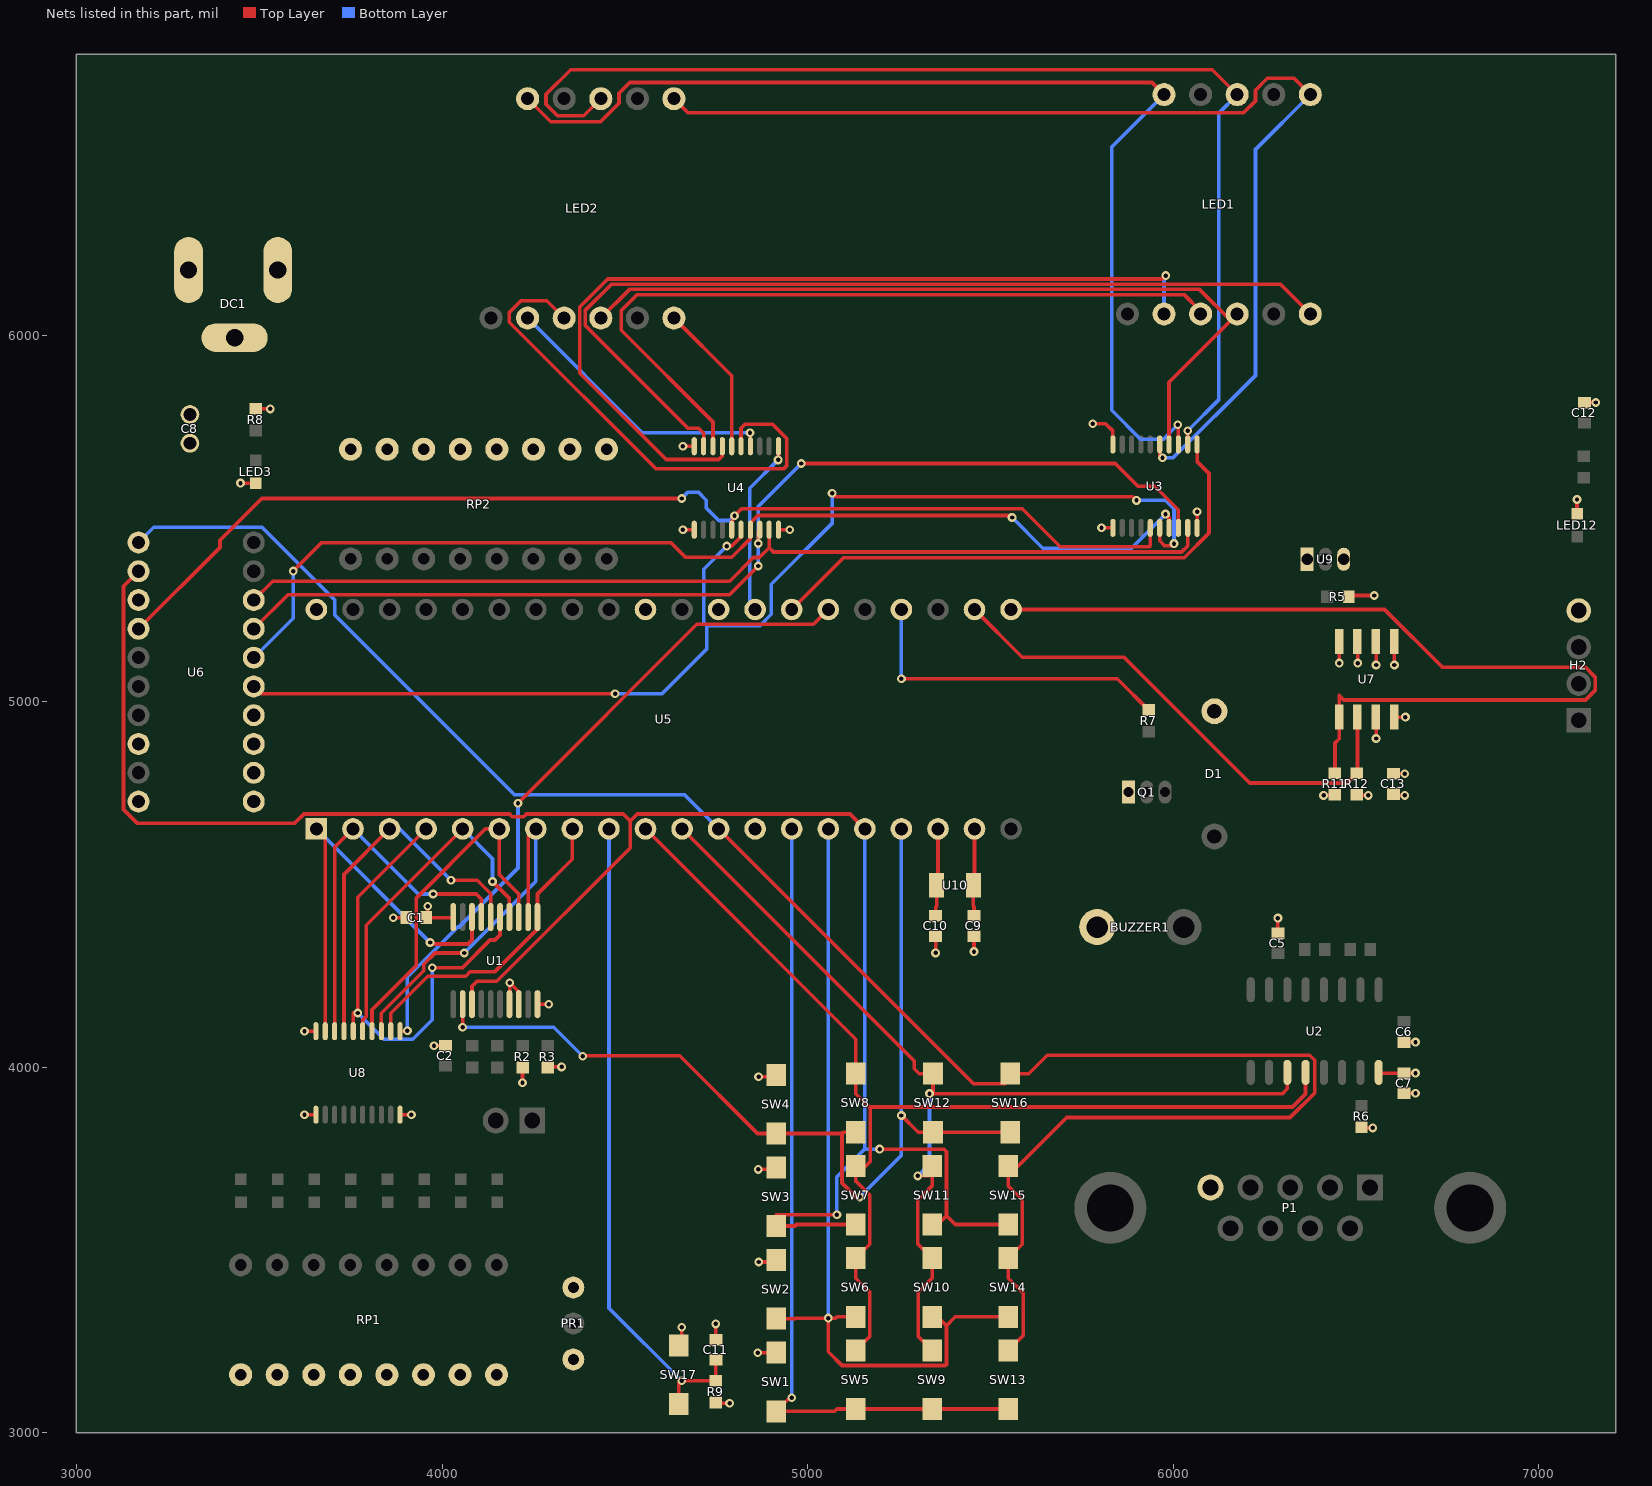
[diagram p0: the nets of this part, all layers, seen from the top]
# Altium PCB MISC49866.pcbdoc (part 2 of 2)
Units mil, origin at the board's own origin, x right, y up, seen from the top; angles counter-clockwise.
Board outline 4210 x 3770 mil, 4 copper layers (Top Layer, Inner1, Inner2, Bottom Layer), stack 62.447 mil thick; 74 components, 100 nets, 357 pads, 104 vias.

## Via types
v1: diameter 24.02, hole 12, Top Layer to Bottom Layer, 104 vias

## Nets (pads, with @x,y where several pads share a name; then routed paths per layer and width w, separated by ;. In a path a pad name is that pad's centre, name@x,y a point inside that pad or via, vN(x,y) a via of type N, cw(c..) or ccw(c..) an arc to the next point about the centre after c; other vN are vias at no path point) (continued)
D3: U3.5 U4.5 U6.4 | length 3125.9
  Top Layer w10: U6.4@3170.04,5198.78 3392.72,5421.46 3392.72,5440.84 3507.3,5555.42 v1(4655.68,5555.42) ; U4.5@4792.36,5470 4792.36,5493.47 4800.03,5501.14 v1(4800.03,5507.98) 4819.15,5527.1 5587.1,5527.1 5691.01,5423.19 5934.85,5423.19 5937.36,5425.7 U3.5@5937.36,5475
  Bottom Layer w10: v1(4655.68,5555.42) 4673.06,5572.8 4700.92,5572.8 4723.08,5550.64 4723.08,5529.42 4757.24,5495.26 4787.31,5495.26 v1(4800.03,5507.98)
D4: U3.6 U4.6 U6.16 | length 3399
  Top Layer w10: U6.16@3485,5041.3 3505.22,5021.08 v1(4473.36,5021.08) ; v1(4779.08,5425.08) 4792.6,5425.08 4817.95,5450.43 U4.6@4817.95,5470 ; v1(5066.96,5569.86) 5076.38,5560.44 5889.43,5560.44 v1(5899.63,5550.16) ; U3.6@5962.95,5475 5962.95,5439.47 5976.72,5425.7 5995.88,5425.7 v1(6002.2,5432.02)
  Bottom Layer w10: v1(4473.36,5021.08) 4601.64,5021.08 4724.33,5143.77 4724.33,5207.49 ; v1(4779.08,5425.08) 4715.87,5361.87 4715.87,5215.95 4724.33,5207.49 ; v1(5066.96,5569.86) 5066.96,5486.96 4900.83,5320.83 4900.83,5238.43 4869.89,5207.49 4724.33,5207.49 ; v1(5899.63,5550.16) 5978.97,5550.16 6002.2,5526.93 v1(6002.2,5432.02)
D5: U3.7 U4.7 U6.15 | length 2905.5
  Top Layer w10: v1(3592.89,5356.8) 3669.98,5433.89 4626.85,5433.89 4665.79,5394.95 4792.72,5394.95 4843.54,5445.77 U4.7@4843.54,5470 4843.54,5488.99 4863.49,5508.94 5553.83,5508.94 v1(5559.36,5503.41) ; v1(5979.04,5512.54) 5988.54,5503.04 U3.7@5988.54,5475
  Bottom Layer w10: U6.15@3485,5120.04 3592.89,5227.93 v1(3592.89,5356.8) ; v1(5559.36,5503.41) 5643.51,5419.26 5885.76,5419.26 v1(5979.04,5512.54)
D6: U3.8 U4.8 U6.14 | length 2953.3
  Top Layer w10: U6.14@3485,5198.78 3578.59,5292.37 4786.35,5292.37 v1(4864.8,5370.82) ; v1(4864.8,5432.12) 4864.8,5465.67 U4.8@4869.13,5470 ; v1(4982.54,5651.13) 5841.27,5651.13 5903.59,5588.81 5949.61,5588.81 6014.13,5524.3 U3.8@6014.13,5475
  Bottom Layer w10: v1(4864.8,5370.82) v1(4864.8,5432.12) 4864.8,5533.4 v1(4982.54,5651.13)
D7: U3.9 U4.9 U6.13 | length 2724.5
  Top Layer w10: U6.13@3485,5277.52 3536.73,5329.25 4786.89,5329.25 4851.62,5393.98 4868,5393.98 4894.72,5420.7 ; U4.9@4894.72,5470 4894.72,5420.7 ; U3.9@6039.72,5475 6039.72,5425.7 6022.88,5408.86 4906.56,5408.86 4894.72,5420.7
DB1: U1.18 U5.1 U8.19 | length 1186.6
  Top Layer w10: U5.1@3656.56,4651.69 3680.59,4627.66 U8.19@3680.59,4098.35 ; v1(3967.37,4340.88) 3971.44,4336.81 4071.19,4336.81 4082.03,4347.65 U1.18@4082.03,4410.54
  Bottom Layer w10: U5.1@3656.56,4651.69 v1(3967.37,4340.88)
DB2: U1.17 U5.2 U8.18 | length 1053.9
  Top Layer w10: U8.18@3706.18,4098.35 3706.18,4601.31 U5.2@3756.56,4651.69 ; v1(3975.6,4473.42) 4093.85,4473.42 4107.62,4459.65 U1.17@4107.62,4410.54
  Bottom Layer w10: U5.2@3756.56,4651.69 3934.83,4473.42 v1(3975.6,4473.42)
DB3: U1.16 U5.3 U8.17 | length 1019.1
  Top Layer w10: U8.17@3731.77,4098.35 3731.77,4526.9 U5.3@3856.56,4651.69 ; v1(4024.51,4511.2) 4096.54,4511.2 4133.21,4474.53 U1.16@4133.21,4410.54
  Bottom Layer w10: U5.3@3856.56,4651.69 3884.02,4651.69 v1(4024.51,4511.2)
DB4: U1.15 U5.4 U8.16 | length 1312.6
  Top Layer w10: U8.16@3757.36,4098.35 3757.36,4147.65 3757.73,4148.02 v1(3769.45,4148.02) 3769.45,4464.58 U5.4@3956.56,4651.69 ; v1(3973.41,4272.07) 4056.01,4272.07 4131.59,4347.65 4145.04,4347.65 4158.81,4361.42 U1.15@4158.8,4410.54
  Bottom Layer w10: v1(3769.45,4148.02) 3841.23,4076.24 3920.25,4076.24 3973.41,4129.4 v1(3973.41,4272.07)
DB5: U1.14 U5.5 U8.15 | length 960.8
  Top Layer w10: U8.15@3782.95,4098.35 3782.95,4128.76 3792.61,4138.42 3792.61,4387.74 U5.5@4056.56,4651.69 ; v1(4138.1,4507.63) 4184.4,4461.34 U1.14@4184.39,4410.54
  Bottom Layer w10: U5.5@4056.56,4651.69 4138.1,4570.15 v1(4138.1,4507.63)
DB6: U1.13 U5.6 U8.14 | length 982.8
  Top Layer w10: U8.14@3808.54,4098.35 3808.54,4157.09 3929.94,4278.49 3929.94,4462.63 4119,4651.69 U5.6@4156.56,4651.69 4156.56,4526.85 4209.98,4473.42 U1.13@4209.98,4410.54
DB7: U1.12 U5.7 U8.13 | length 1025
  Top Layer w10: U8.13@3834.13,4098.35 3834.13,4147.65 3950.25,4263.77 3950.25,4281.66 3980.86,4312.27 v1(4060.88,4312.27) ; U1.12@4235.57,4410.54 4235.57,4630.71 U5.7@4256.56,4651.69
  Bottom Layer w10: v1(4060.88,4312.27) 4256.55,4507.95 U5.7@4256.56,4651.69
DB8: U1.11 U5.8 U8.12 | length 859.5
  Top Layer w10: U8.12@3859.72,4098.35 3859.72,4147.65 3960.98,4248.91 4064.81,4248.91 4077.24,4261.34 4144.77,4261.34 4261.16,4377.74 U1.11@4261.16,4410.54 4261.16,4473.42 4356.55,4568.81 U5.8@4356.56,4651.69
DIOLA: U5.26 U8.11 | length 1838.5
  Top Layer w10: U8.11@3885.32,4098.35 3904.19,4098.35 v1(3905.25,4099.41) ; v1(4207.78,4721.97) 4696.82,5211.01 5015.87,5211.01 U5.26@5056.56,5251.69
  Bottom Layer w10: v1(3905.25,4099.41) 3905.25,4245.6 4042.78,4383.13 4046.38,4383.13 4207.78,4544.54 v1(4207.78,4721.97)
DP: LED1.3 LED2.3 U3.12 | length 3169
  Top Layer w10: LED2.3@4434.27,6648.78 4387.67,6602.18 4315.93,6602.18 4284.27,6633.84 4284.27,6660.64 4351.96,6728.33 6106.67,6728.33 LED1.3@6175,6660 ; U3.12@6039.72,5703.35 v1(6039.72,5740.75)
  Bottom Layer w10: v1(6039.72,5740.75) 6125,5826.03 6125,6610 LED1.3@6175,6660
DULA: U3.11 U5.27 | length 1484
  Top Layer w10: U5.27@4956.56,5251.69 5098.28,5393.42 6030.27,5393.42 6098.02,5461.17 6098.02,5623.77 6065.32,5656.46 U3.11@6065.31,5703.35
E: LED1.1 LED2.1 U3.15 | length 3049.5
  Top Layer w10: LED2.1@4634.27,6648.78 4672.89,6610.16 6192.41,6610.16 6225,6642.75 6225,6672.1 6257.49,6704.59 6330.41,6704.59 LED1.1@6375,6660 ; U3.15@5962.95,5703.35 5962.95,5674.2 v1(5970.66,5666.49)
  Bottom Layer w10: v1(5970.66,5666.49) 5999.7,5666.49 6225,5891.79 6225,6510 LED1.1@6375,6660
F: LED1.10 LED2.10 U3.14 | length 2224.5
  Top Layer w10: LED2.10@4434.27,6048.78 4512.74,6127.25 6071.97,6127.25 LED1.10@6157.11,6042.11 ; U3.14@5988.54,5703.35 5988.54,5873.54 LED1.10@6157.11,6042.11 ; LED1.10@6175,6060 LED1.10@6157.11,6042.11
G: LED1.5 LED2.5 U3.13 | length 3047.6
  Top Layer w10: LED2.5@4234.27,6648.78 4297.18,6585.87 4433.53,6585.87 4484.27,6636.61 4484.27,6663.98 4513.23,6692.94 5942.06,6692.94 LED1.5@5975,6660 ; v1(6012.23,5756.74) 6014.13,5754.84 U3.13@6014.13,5703.35
  Bottom Layer w10: LED1.5@5975,6660 5831.75,6516.75 5831.75,5796.71 5911.5,5716.96 5972.45,5716.96 v1(6012.23,5756.74)
GND: BUZZER1.1 C1.2 C2.2 C5.1 C7.1 C8.2 C9.1 C10.1 C13.2 D1.2 DC1.2 DC1.3 H2.4 LED3.1 LED12.1 P1.5 PR1.3 R2.2 R6.1 R9.1 SW1.1 SW2.1 SW3.1 SW4.1 U1.7 U1.8 U1.10 U3.1 U3.10 U4.1 U4.10 U6.3 U6.10 U6.17 U6.18 U7.1 U7.2 U7.3 U7.4 U7.7 U8.1 U8.10 U9.1 | length 1092.7
  Top Layer w10: v1(3448.77,5597.33) LED3.1@3479.81,5597.33 ; v1(3623.96,3870) U8.1@3655,3870 ; v1(3866.74,4408.78) C1.2@3897.78,4408.78 ; U8.10@3885.32,3870 v1(3916.35,3870) ; v1(3978.24,4058.53) C2.2@4009.27,4058.53 ; U1.7@4185,4200 v1(4185,4231.04) 4209.98,4206.06 U1.8@4209.98,4172.03 ; v1(4220.26,3956.99) R2.2@4220.26,3988.02 ; U1.10@4261.16,4172.03 v1(4292.2,4172.03) ; v1(4658.96,5470) U4.1@4690,5470 ; R9.1@4755.61,3080.73 v1(4786.65,3080.73) ; v1(4863.91,3218.9) SW1.1@4894.95,3218.9 ; v1(4865.29,3720.25) SW3.1@4896.32,3720.25 ; v1(4865.84,3973.59) SW4.1@4896.87,3973.59 ; v1(4866.39,3466.92) SW2.1@4897.42,3466.92 ; U4.10@4920.31,5470 v1(4951.35,5470) ; v1(5350.03,4312.48) C10.1@5350.03,4343.52 ; v1(5455.03,4316.1) C9.1@5455.03,4347.13 ; v1(5803.96,5475) U3.1@5835,5475 ; U3.10@6065.31,5488.28 v1(6065.31,5519.32) ; C5.1@6286.36,4376.51 v1(6286.36,4407.55) ; v1(6453.96,5105) U7.4@6453.96,5164.04 ; U7.3@6503.96,5164.04 6505,5163.01 v1(6505,5105) ; R6.1@6515,3833.7 v1(6546.04,3833.7) ; U7.2@6553.96,5164.04 6555,5163.01 v1(6555,5100) ; v1(6555,4898.96) U7.7@6555,4930 ; C13.2@6602.32,4743.12 v1(6633.36,4743.12) ; U7.1@6603.96,5164.04 6605,5163.01 v1(6605,5100) ; C7.1@6631.76,3928.55 v1(6662.79,3928.55) ; LED12.1@7104.55,5521.5 v1(7104.55,5552.53)
INT0: SW13.2 SW14.2 SW15.2 SW16.2 U5.12 U6.1 | length 5525.8
  Top Layer w10: U5.12@4756.56,4651.69 5453.44,3954.8 5540.16,3954.8 5553.93,3968.57 SW16.2@5553.93,3982.11 5605.2,3982.11 5655.48,4032.39 6373.36,4032.39 6387.02,4018.73 6387.02,3929.49 6319.62,3862.09 5708.59,3862.09 SW15.2@5548.93,3702.43 ; SW13.2@5548.93,3224.99 5589.64,3265.7 5589.64,3382.03 5548.93,3422.74 SW14.2@5548.93,3477.36 5586.85,3515.28 5586.85,3637.2 5548.93,3675.12 SW15.2@5548.93,3702.43 ; SW15.2@5548.93,3729.74 SW15.2@5548.93,3702.43
  Bottom Layer w10: U6.1@3170.04,5435 3211.83,5476.79 3507.58,5476.79 3706.56,5277.81 3706.56,5236.77 4198.19,4745.13 4663.11,4745.13 U5.12@4756.56,4651.69
INT1: U5.13
LCDEN: SW1.2 SW5.1 SW9.1 SW13.1 U5.14 | length 2250.8
  Top Layer w10: v1(4956.55,3095.68) 4951.29,3095.68 SW1.2@4914.27,3058.66 5074.59,3058.66 5080.68,3064.75 5131.95,3064.75 5340.44,3064.75 SW13.1@5548.93,3064.75
  Bottom Layer w10: v1(4956.55,3095.68) U5.14@4956.56,4651.69
M11: LED1.12 U4.19 | length 2569.5
  Top Layer w10: U4.19@4715.59,5698.35 4715.59,5733.87 4701.82,5747.64 4672.95,5747.64 4391.37,6029.22 4391.37,6069.43 4463.38,6141.44 6293.56,6141.44 LED1.12@6375,6060
M12: LED1.9 U4.18 | length 2103.8
  Top Layer w10: U4.18@4741.18,5698.35 4741.18,5764.5 4490.54,6015.14 4490.54,6069.4 4534.2,6113.06 6029.42,6113.06 6075,6067.48 LED1.9@6075,6060
M13: LED1.8 U4.17 | length 2444.4
  Top Layer w10: U4.17@4766.77,5698.35 4766.77,5671.42 4757.29,5661.94 4613.06,5661.94 4376.91,5898.09 4376.91,6079.04 4453.5,6155.63 5970.06,6155.63 v1(5979.41,6164.98)
  Bottom Layer w10: LED1.8@5975,6060 5975,6160.57 v1(5979.41,6164.98)
M21: LED2.12 U4.16 | length 415.9
  Top Layer w10: LED2.12@4634.27,6048.78 4792.36,5890.69 U4.16@4792.36,5698.35
M22: LED2.9 U4.15 | length 1406.8
  Top Layer w10: LED2.9@4334.27,6048.78 4286.84,6096.21 4216.23,6096.21 4184.27,6064.25 4184.27,6037.16 4584.34,5637.09 4935.34,5637.09 4942.48,5644.23 4942.48,5719.88 4903.87,5758.49 4828.8,5758.49 4817.95,5747.64 U4.15@4817.95,5698.35
M23: LED2.8 U4.14 | length 775.4
  Top Layer w10: v1(4842.41,5735.33) 4843.54,5734.2 U4.14@4843.54,5698.35
  Bottom Layer w10: LED2.8@4234.27,6048.78 4547.72,5735.33 v1(4842.41,5735.33)
P30: SW5.2 SW6.2 SW7.2 SW8.2 U2.12 U5.10 | length 3053.3
  Top Layer w10: U5.10@4556.56,4651.69 5131.95,4076.29 SW8.2@5131.95,3982.11 5131.95,3927.49 5171.17,3888.27 ; SW5.2@5131.95,3224.99 5169.87,3262.91 5169.87,3384.82 5131.95,3422.74 SW6.2@5131.95,3477.36 5169.87,3515.28 5169.87,3650.45 5131.95,3688.36 SW7.2@5131.95,3702.43 ; SW7.2@5131.95,3729.74 SW7.2@5131.95,3702.43 ; U2.12@6362.02,3985.58 6362.02,3926.73 6326.08,3890.79 5173.69,3890.79 5171.17,3888.27 ; SW7.2@5131.95,3702.43 5171.17,3741.65 5171.17,3888.27
P31: SW9.2 SW10.2 SW11.2 SW12.2 U2.11 U5.11 | length 2906.5
  Top Layer w10: U5.11@4656.56,4651.69 5291.67,4016.57 5291.67,3995.88 5305.44,3982.11 SW12.2@5342.94,3982.11 v1@5342.94,3927.49 ; v1(5301.05,3702.43) SW11.2@5340.44,3702.43 ; v1(5333.54,3927.49) v1@5342.94,3927.49 ; SW9.2@5340.44,3224.99 5302.52,3262.91 5302.52,3384.82 5340.44,3422.74 SW10.2@5340.44,3477.36 5301.35,3516.45 5301.35,3636.03 5340.44,3675.12 SW11.2@5340.44,3702.43 ; SW11.2@5340.44,3729.74 SW11.2@5340.44,3702.43 ; U2.11@6312.02,3985.58 6312.02,3940.5 6298.25,3926.73 5343.7,3926.73 v1@5342.94,3927.49
  Bottom Layer w10: v1(5301.05,3702.43) 5333.54,3734.92 v1(5333.54,3927.49)
PSEN: U5.29
RD: SW4.2 SW8.1 SW12.1 SW16.1 U1.2 U5.17 | length 2830.8
  Top Layer w10: v1(4056.44,4109.14) U1.2@4056.44,4172.03 ; v1@4385,4031.41 4650.25,4031.41 4863,3818.66 SW4.2@4914.27,3818.66 5094.03,3818.66 ; SW8.1@5131.95,3821.87 5097.24,3821.87 5094.03,3818.66 ; v1(5142.6,3644.96) 5132.19,3644.96 5094.03,3683.12 5094.03,3818.66 ; v1(5256.55,3867.63) 5302.3,3821.87 SW12.1@5342.94,3821.87 SW16.1@5553.93,3821.87
  Bottom Layer w10: v1(4056.44,4109.14) 4305.86,4109.14 v1(4385,4030) ; v1(5142.6,3644.96) 5256.55,3758.91 v1(5256.55,3867.63) U5.17@5256.56,4651.69
RS: SW2.2 SW6.1 SW10.1 SW14.1 U5.15 | length 2324.9
  Top Layer w10: SW2.2@4914.27,3312 4965.54,3311.99 4967.13,3313.58 v1(5056.55,3313.58) ; SW6.1@5131.95,3317.12 5080.68,3317.12 5077.14,3313.58 v1(5056.55,3313.58) ; SW10.1@5340.44,3317.12 5355.44,3317.12 5379.74,3292.82 ; SW14.1@5548.93,3317.12 5404.04,3317.12 5379.74,3292.82 ; v1(5056.55,3313.58) 5056.55,3221.34 5094.17,3183.72 5376.83,3183.72 5379.74,3186.63 5379.74,3292.82
  Bottom Layer w10: v1(5056.55,3313.58) U5.15@5056.56,4651.69
RST: C11.1 R9.2 SW17.2 U5.9 | length 1809.8
  Top Layer w10: SW17.2@4647.12,3078.9 4647.11,3133.52 v1(4655.48,3141.89) R9.2@4748.84,3141.89 C11.1@4748.84,3199.67
  Bottom Layer w10: U5.9@4456.56,4651.69 4456.55,3340.82 v1(4655.48,3141.89)
SCL: R12.1 U5.22 U7.6 | length 1407.2
  Top Layer w10: U5.22@5456.56,5251.69 5587.38,5120.87 5865.67,5120.87 6209.29,4777.25 6475.29,4777.25 R12.1@6502.32,4804.28 6503.96,4805.92 U7.6@6503.96,4957.32
SDA: R11.1 U5.21 U7.5 | length 2643.3
  Top Layer w10: U5.21@5556.56,5251.69 6578.14,5251.69 6736.44,5093.39 7127.76,5093.39 7153.89,5067.26 7153.89,5030.3 7127.76,5004.17 6466.08,5004.17 6453.96,5016.29 U7.5@6453.96,4957.32 6453.96,4898.37 6442.32,4886.73 R11.1@6442.32,4804.28
SPK: R7.1 U5.24 | length 900.8
  Top Layer w10: v1(5256.55,5062.53) 5846.97,5062.53 R7.1@5932.67,4976.83
  Bottom Layer w10: v1(5256.55,5062.53) U5.24@5256.56,5251.69
VCC: C1.1 C6.1 C7.2 C8.1 C11.2 C12.2 C13.1 DC1.1 PR1.1 Q1.1 R3.1 R5.2 R8.2 R11.2 R12.2 RP1.1 RP1.2 RP1.3 RP1.4 RP1.5 RP1.6 RP1.7 RP1.8 RP2.9 RP2.10 RP2.11 RP2.12 RP2.13 RP2.14 RP2.15 RP2.16 SW17.1 U1.20 U2.16 U3.20 U4.20 U5.31 U5.40 U6.8 U6.19 U6.20 U7.8 U8.20 U9.3 | length 759.5
  Top Layer w10: R8.2@3490.61,5800.49 v1(3530,5800.49) ; v1(3623.96,4098.35) U8.20@3655,4098.35 ; C1.1@3956.83,4408.78 C1.1@3960.77,4408.78 ; v1(3960.77,4439.82) C1.1@3960.77,4408.78 ; U1.20@4030.85,4410.54 4029.09,4408.78 C1.1@3960.77,4408.78 ; R3.1@4296.04,4000.63 v1(4327.08,4000.63) ; SW17.1@4655.59,3257.45 v1(4655.59,3288.48) ; v1(4658.96,5698.35) U4.20@4690,5698.35 ; C11.2@4748.84,3266.68 v1(4748.84,3297.72) ; v1(5780,5760) 5815,5760 5835,5740 U3.20@5835,5703.35 ; v1(6411.28,4743.32) R11.2@6442.32,4743.32 ; R5.2@6479.91,5286.78 6483.13,5290 v1(6550,5290) ; R12.2@6502.32,4743.32 v1(6533.36,4743.32) ; U2.16@6562.02,3985.58 6563.93,3983.67 C7.2@6631.76,3983.67 v1(6662.79,3983.67) ; C13.1@6602.32,4802.18 v1(6633.36,4802.18) ; U7.8@6603.96,4957.32 v1(6635,4957.32) ; C6.1@6631.76,4068.55 v1(6662.79,4068.55) ; C12.2@7124.88,5817.81 v1(7155.92,5817.81)
WELA: U4.11 U5.28 | length 485.5
  Top Layer w10: v1(4919.26,5660.8) 4920.32,5661.86 U4.11@4920.31,5698.35
  Bottom Layer w10: U5.28@4856.56,5251.69 4841.56,5266.68 4841.56,5583.1 v1(4919.26,5660.8)
WR: SW3.2 SW7.1 SW11.1 SW15.1 U1.3 U5.16 U6.2 | length 5606.3
  Top Layer w10: U6.2@3170.04,5356.26 3128.77,5314.99 3128.77,4704.46 3165.71,4667.52 3597.57,4667.52 3622.42,4692.37 4184.56,4692.37 4192.31,4684.62 4223.26,4684.62 4231.01,4692.37 4495.62,4692.37 4514.61,4673.38 ; U1.3@4082.03,4172.03 4082.03,4221.14 4095.8,4234.91 4149.93,4234.91 4514.61,4599.6 4514.61,4673.38 ; v1(5080,3595.98) 4914.51,3595.98 4914.27,3595.74 SW3.2@4914.27,3565.33 4965.54,3565.33 4969.71,3569.5 SW7.1@5131.95,3569.5 ; U5.16@5156.56,4651.69 5115.78,4692.46 4533.69,4692.46 4514.61,4673.38 ; v1(5196.89,3775.81) 5372.55,3775.81 5379.71,3768.65 5379.71,3593.77 ; SW11.1@5340.44,3569.5 5355.44,3569.5 5379.71,3593.77 ; SW15.1@5548.93,3569.5 5403.98,3569.5 5379.71,3593.77
  Bottom Layer w10: v1(5080,3595.98) 5080,3699.26 5156.55,3775.81 ; U5.16@5156.56,4651.69 5156.55,3775.81 ; v1(5196.89,3775.81) 5156.55,3775.81
XTAL1: C9.2 U5.19 U10.2 | length 269
  Top Layer w10: U10.2@5453.44,4497.68 U10.2@5453.44,4468.71 ; C9.2@5455.03,4413.6 5455.03,4438.14 5453.44,4439.73 U10.2@5453.44,4468.71 ; U5.19@5456.56,4651.69 5456.56,4471.83 U10.2@5453.44,4468.71
XTAL2: C10.2 U5.18 U10.1 | length 269.8
  Top Layer w10: C10.2@5350.03,4413.6 5350.03,4436.72 5353.04,4439.73 U10.1@5353.04,4468.71 ; U10.1@5353.04,4497.68 U10.1@5353.04,4468.71 ; U5.18@5356.56,4651.69 5356.56,4472.23 U10.1@5353.04,4468.71
pads on no net: P1.1 P1.4 P1.6 P1.7 P1.8 P1.9 P1.10 P1.11 U1.5 U2.7 U2.8 U2.9 U2.10 U4.12 U4.13 U5.20

## Keep-outs
Board Outline Layer:
  region: 3208.22,6645 cw(c3125,6645) 3041.78,6645 cw(c3125,6645)
  circle w0.1: c3125,6645 r83.22
  region: 3208.22,6645 3207.84,6637.09 3206.71,6629.25 3204.85,6621.56 3202.26,6614.07 3198.97,6606.87 3195.01,6600.01 3190.41,6593.56 3185.23,6587.57 3179.5,6582.11 3173.27,6577.21 3166.61,6572.93 3159.57,6569.3 3152.22,6566.36 3144.62,6564.13 3136.84,6562.63 3128.96,6561.88 3121.04,6561.88 3113.16,6562.63 3105.38,6564.13 3097.78,6566.36 3090.43,6569.3 3083.39,6572.93 3076.73,6577.21 3070.5,6582.11 3064.77,6587.57 3059.59,6593.56 3054.99,6600.01 3051.03,6606.87 3047.74,6614.07 3045.15,6621.56 3043.29,6629.25 3042.16,6637.09 3041.78,6645 3042.16,6652.91 3043.29,6660.75 3045.15,6668.44 3047.74,6675.93 3051.03,6683.13 3054.99,6689.99 3059.59,6696.44 3064.77,6702.43 3070.5,6707.89 3076.73,6712.79 3083.39,6717.07 3090.43,6720.7 3097.78,6723.64 3105.38,6725.87 3113.16,6727.37 3121.04,6728.12 3128.96,6728.12 3136.84,6727.37 3144.62,6725.87 3152.22,6723.64 3159.57,6720.7 3166.61,6717.07 3173.27,6712.79 3179.5,6707.89 3185.23,6702.43 3190.41,6696.44 3195.01,6689.99 3198.97,6683.13 3202.26,6675.93 3204.85,6668.44 3206.71,6660.75 3207.84,6652.91
  region: 7168.22,6645 cw(c7085,6645) 7001.78,6645 cw(c7085,6645)
  circle w0.1: c7085,6645 r83.22
  region: 7168.22,6645 7167.84,6637.09 7166.71,6629.25 7164.85,6621.56 7162.26,6614.07 7158.97,6606.87 7155.01,6600.01 7150.41,6593.56 7145.23,6587.57 7139.5,6582.11 7133.27,6577.21 7126.61,6572.93 7119.57,6569.3 7112.22,6566.36 7104.62,6564.13 7096.84,6562.63 7088.96,6561.88 7081.04,6561.88 7073.16,6562.63 7065.38,6564.13 7057.78,6566.36 7050.43,6569.3 7043.39,6572.93 7036.73,6577.21 7030.5,6582.11 7024.77,6587.57 7019.59,6593.56 7014.99,6600.01 7011.03,6606.87 7007.74,6614.07 7005.15,6621.56 7003.29,6629.25 7002.16,6637.09 7001.78,6645 7002.16,6652.91 7003.29,6660.75 7005.15,6668.44 7007.74,6675.93 7011.03,6683.13 7014.99,6689.99 7019.59,6696.44 7024.77,6702.43 7030.5,6707.89 7036.73,6712.79 7043.39,6717.07 7050.43,6720.7 7057.78,6723.64 7065.38,6725.87 7073.16,6727.37 7081.04,6728.12 7088.96,6728.12 7096.84,6727.37 7104.62,6725.87 7112.22,6723.64 7119.57,6720.7 7126.61,6717.07 7133.27,6712.79 7139.5,6707.89 7145.23,6702.43 7150.41,6696.44 7155.01,6689.99 7158.97,6683.13 7162.26,6675.93 7164.85,6668.44 7166.71,6660.75 7167.84,6652.91
  region: 7168.22,3125 cw(c7085,3125) 7001.78,3125 cw(c7085,3125)
  circle w0.1: c7085,3125 r83.22
  region: 7168.22,3125 7167.84,3117.09 7166.71,3109.25 7164.85,3101.56 7162.26,3094.07 7158.97,3086.87 7155.01,3080.01 7150.41,3073.56 7145.23,3067.57 7139.5,3062.11 7133.27,3057.21 7126.61,3052.93 7119.57,3049.3 7112.22,3046.36 7104.62,3044.13 7096.84,3042.63 7088.96,3041.88 7081.04,3041.88 7073.16,3042.63 7065.38,3044.13 7057.78,3046.36 7050.43,3049.3 7043.39,3052.93 7036.73,3057.21 7030.5,3062.11 7024.77,3067.57 7019.59,3073.56 7014.99,3080.01 7011.03,3086.87 7007.74,3094.07 7005.15,3101.56 7003.29,3109.25 7002.16,3117.09 7001.78,3125 7002.16,3132.91 7003.29,3140.75 7005.15,3148.44 7007.74,3155.93 7011.03,3163.13 7014.99,3169.99 7019.59,3176.44 7024.77,3182.43 7030.5,3187.89 7036.73,3192.79 7043.39,3197.07 7050.43,3200.7 7057.78,3203.64 7065.38,3205.87 7073.16,3207.37 7081.04,3208.12 7088.96,3208.12 7096.84,3207.37 7104.62,3205.87 7112.22,3203.64 7119.57,3200.7 7126.61,3197.07 7133.27,3192.79 7139.5,3187.89 7145.23,3182.43 7150.41,3176.44 7155.01,3169.99 7158.97,3163.13 7162.26,3155.93 7164.85,3148.44 7166.71,3140.75 7167.84,3132.91
  region: 3208.22,3125 cw(c3125,3125) 3041.78,3125 cw(c3125,3125)
  circle w0.1: c3125,3125 r83.22
  region: 3208.22,3125 3207.84,3117.09 3206.71,3109.25 3204.85,3101.56 3202.26,3094.07 3198.97,3086.87 3195.01,3080.01 3190.41,3073.56 3185.23,3067.57 3179.5,3062.11 3173.27,3057.21 3166.61,3052.93 3159.57,3049.3 3152.22,3046.36 3144.62,3044.13 3136.84,3042.63 3128.96,3041.88 3121.04,3041.88 3113.16,3042.63 3105.38,3044.13 3097.78,3046.36 3090.43,3049.3 3083.39,3052.93 3076.73,3057.21 3070.5,3062.11 3064.77,3067.57 3059.59,3073.56 3054.99,3080.01 3051.03,3086.87 3047.74,3094.07 3045.15,3101.56 3043.29,3109.25 3042.16,3117.09 3041.78,3125 3042.16,3132.91 3043.29,3140.75 3045.15,3148.44 3047.74,3155.93 3051.03,3163.13 3054.99,3169.99 3059.59,3176.44 3064.77,3182.43 3070.5,3187.89 3076.73,3192.79 3083.39,3197.07 3090.43,3200.7 3097.78,3203.64 3105.38,3205.87 3113.16,3207.37 3121.04,3208.12 3128.96,3208.12 3136.84,3207.37 3144.62,3205.87 3152.22,3203.64 3159.57,3200.7 3166.61,3197.07 3173.27,3192.79 3179.5,3187.89 3185.23,3182.43 3190.41,3176.44 3195.01,3169.99 3198.97,3163.13 3202.26,3155.93 3204.85,3148.44 3206.71,3140.75 3207.84,3132.91
  lines w10: 3000,3000 3000,6770 7210,6770 7210,3000 3000,3000

## Silkscreen, mask and mechanical layers (free items; w line width, h text height)
Mechanical Layer:
  circle w0.1: c3125,6645 r83.22
  circle w0.1: c7085,6645 r83.22
  circle w0.1: c7085,3125 r83.22
  circle w0.1: c3125,3125 r83.22